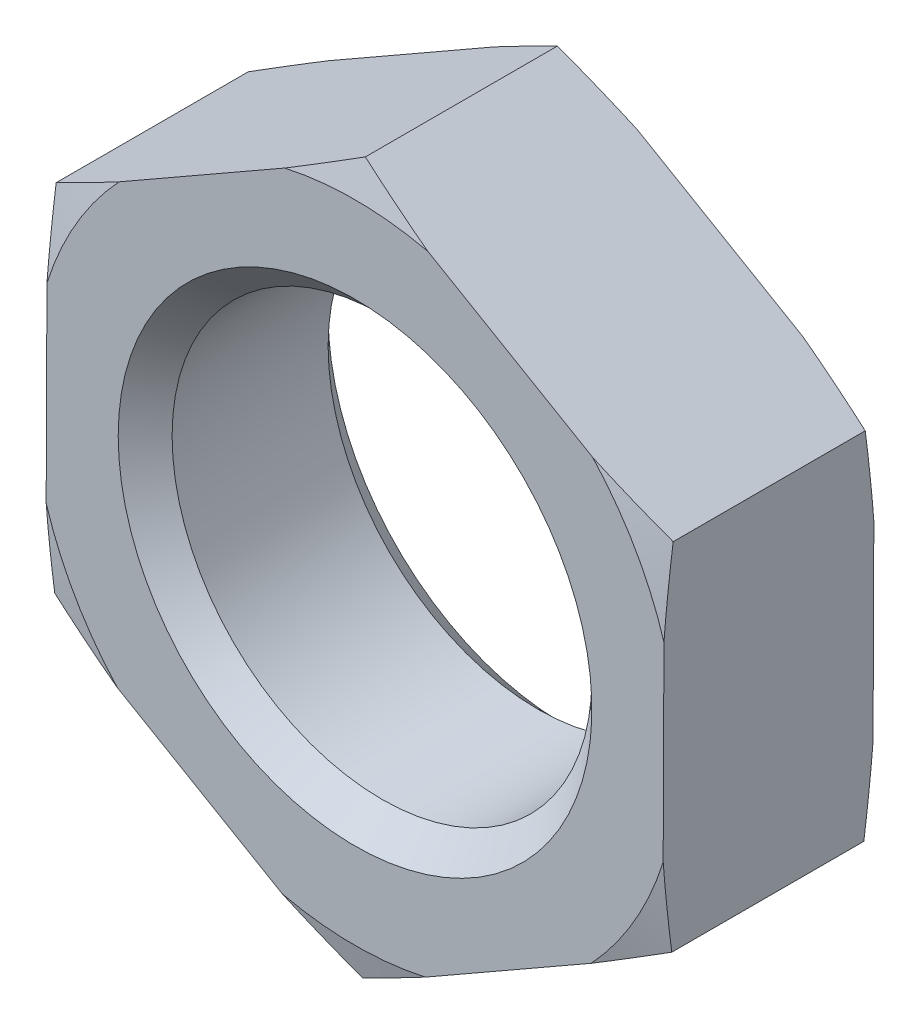
SolidWorks part; units mm, degrees
extrude "Base-Extrude" add sketch "Sketch1" along normal blind 26
sketch "Sketch1" plane through (0, 0, 0) normal (0, 0, 1) x (1, 0, 0)
  line L0 (-26.8088, 0) -> (37.1748, 0) construction
  line L1 (0, 25.0215) -> (0, -25.0215) construction
  line L3 (0.1736, 44.1247) -> (-38.1263, 22.2126)
  line L4 (-38.1263, 22.2126) -> (-38.2999, -21.912)
  line L5 (-38.2999, -21.912) -> (-0.1736, -44.1247)
  line L6 (-0.1736, -44.1247) -> (38.1263, -22.2126)
  line L7 (38.1263, -22.2126) -> (38.2999, 21.912)
  line L8 (38.2999, 21.912) -> (0.1736, 44.1247)
  circle A0 centre (0, 0) radius 38.2134 construction
  circle A1 centre (0, 0) radius 26
cosmetic thread "Cosmetic Thread1"
chamfer "Chamfer1" distance 3.3381 angle 45 2 edges at (26, 0, 0) (26, 0, 26)
material "04级"
ref_plane "Plane1" through (0, 0, 0) normal (0, 0, 1) x (1, 0, 0)
ref_plane "Plane2" through (0, 0, 0) normal (0, 1, 0) x (1, 0, 0)
ref_plane "Plane3" through (0, 0, 0) normal (1, 0, 0) x (0, 0, -1)
sketch "Dimension sketch" plane through (0, 0, 0) normal (0, 0, 1) x (1, 0, 0)
  line L0 (0, 0) -> (24.1005, 0)
  line L1 (0, 0) -> (56.2, 0)
  line L2 (46.8781, 0) -> (121.0781, 0)
  line L3 (-49.5238, 0) -> (0, 0)
  point P3 (52, 0)
  point P4 (2.5, 0)
  point P5 (88.25, 0)
  point P6 (26, 0)
  point P7 (7.3, 0)
  point P8 (80, 0)
sketch "Sketch2" plane through (0, 0, 0) normal (0, 0, -1) x (-1, 0, 0)
  circle A0 centre (0, 0) radius 40
  circle A1 centre (0, 0) radius 26 construction
extrude "Cut-Extrude1" cut sketch "Sketch2" against normal through all draft 75 flip side to cut
sketch "Sketch3" plane through (0, 0, 26) normal (0, 0, 1) x (1, 0, 0)
  circle A0 centre (0, 0) radius 40
extrude "Cut-Extrude2" cut sketch "Sketch3" against normal through all draft 75 flip side to cut
equation "\"e@Sketch1\" = \"e@Dimension sketch\""
equation "\"D1@Dimension sketch\" = \"D@Dimension sketch\" / 1.05"
equation "\"D@Sketch1\" = \"D@Dimension sketch\""
equation "\"m@Base-Extrude\" = \"m@Dimension sketch\""
equation "\"D1@Sketch3\" = \"s@Dimension sketch\""
equation "\"s@Sketch2\" = \"s@Dimension sketch\""
equation "\"D2@Cosmetic Thread1\" = 1.05 * \"D1@Dimension sketch\""
equation "\"D1@Chamfer1\" =  ( \"da@Dimension sketch\" - \"D1@Dimension sketch\" )  / 2"
